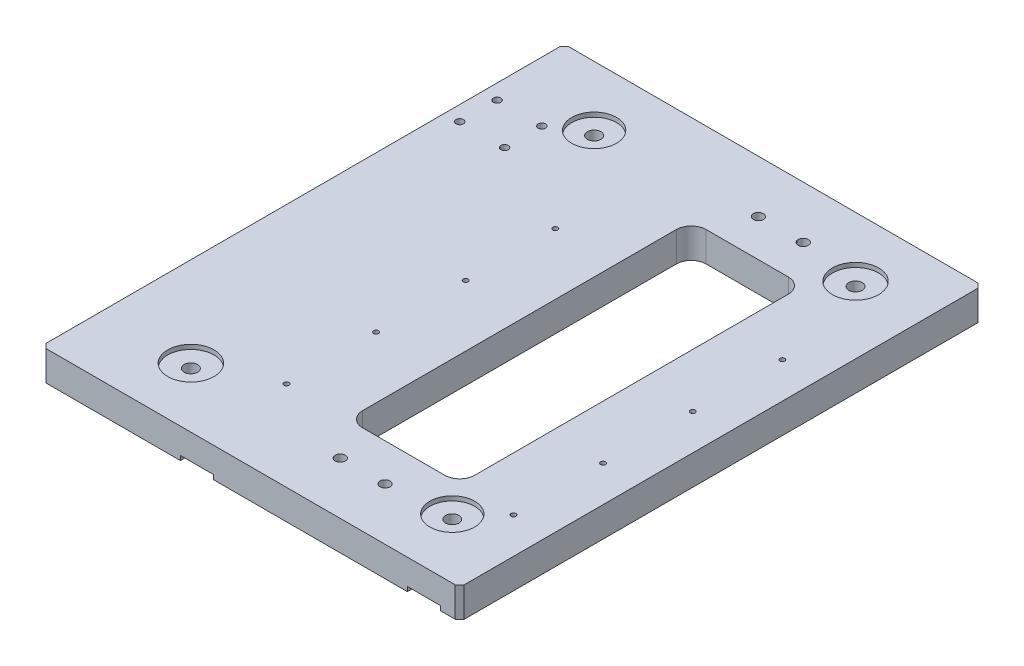
from build123d import *

# Parameters (mm, degrees)
BOSS_EXTRUDE1_DEPTH         = 350
CHAMFER1_SIZE               = 3
SKETCH2_W                   = 75
SKETCH2_H                   = 230
CUT_EXTRUDE1_DEPTH          = 395.884460879
FILLET1_R                   = 10
HOLE1_D                     = 9
HOLE1_DEPTH                 = 17
HOLE1_CBORE_D               = 15
HOLE1_CBORE_DEPTH           = 10.5
M4_TAPPED_HOLE1_D           = 3.3
M4_TAPPED_HOLE1_CSINK_D     = 4.05
M4_TAPPED_HOLE1_CSINK_ANGLE = 90
HOLE2_D                     = 31
HOLE2_DEPTH                 = 3
HOLE3_D                     = 30
HOLE3_DEPTH                 = 3
M8_TAPPED_HOLE1_D           = 6.8
M6_TAPPED_HOLE2_D           = 5


with BuildPart() as part:
    # Sketch1 → Boss-Extrude1 (new body)
    with BuildSketch(Plane.XY):
        Polygon((16.751856783, 37.381546135), (146.751856783, 37.381546135), (146.751856783, 40.381546135), (168.751856783, 40.381546135), (168.751856783, 37.381546135), (181.751856783, 37.381546135), (181.751856783, 57.381546135), (-98.248143217, 57.381546135), (-98.248143217, 37.381546135), (-5.248143217, 37.381546135), (-5.248143217, 40.381546135), (16.751856783, 40.381546135), align=None)
    extrude(amount=BOSS_EXTRUDE1_DEPTH)

    # Chamfer1
    chamfer1_edges = [part.edges().sort_by_distance(p)[0] for p in [
        (181.751856783, 47.381546135, 0),
        (-98.248143217, 47.381546135, 0),
        (181.751856783, 47.381546135, 350),
        (-98.248143217, 47.381546135, 350),
    ]]
    chamfer(chamfer1_edges, length=CHAMFER1_SIZE)

    # Sketch2 → Cut-Extrude1 (cut, through all)
    with BuildSketch(Plane.XZ.offset(-37.381546135)):
        with Locations((84.251856783, 175)):
            Rectangle(SKETCH2_W, SKETCH2_H)
    extrude(amount=-CUT_EXTRUDE1_DEPTH, mode=Mode.SUBTRACT)

    # Fillet1
    fillet1_edges = [part.edges().sort_by_distance(p)[0] for p in [
        (46.751856783, 47.381546135, 60),
        (46.751856783, 47.381546135, 290),
        (121.751856783, 47.381546135, 290),
        (121.751856783, 47.381546135, 60),
    ]]
    fillet(fillet1_edges, radius=FILLET1_R)

    # Hole1
    with Locations(Plane(origin=(0, 37.381546135, 0), x_dir=(-1, 0, 0), z_dir=(0, -1, 0))):
        with Locations((38.248143217, -310), (-136.751856783, -310), (-136.751856783, -40), (38.248143217, -40)):
            CounterBoreHole(HOLE1_D / 2, HOLE1_CBORE_D / 2, HOLE1_CBORE_DEPTH, depth=HOLE1_DEPTH)

    # M4 Tapped Hole1 (through all)
    with Locations(Plane(origin=(0, 40.381546135, 0), x_dir=(-1, 0, 0), z_dir=(0, -1, 0))):
        with Locations((-5.751856783, -290), (-5.751856783, -230), (-5.751856783, -170), (-157.751856783, -170), (-157.751856783, -230), (-157.751856783, -290), (-5.751856783, -110), (-157.751856783, -110)):
            CounterSinkHole(M4_TAPPED_HOLE1_D / 2, M4_TAPPED_HOLE1_CSINK_D / 2, counter_sink_angle=M4_TAPPED_HOLE1_CSINK_ANGLE)

    # Hole2
    with Locations(Plane(origin=(0, 57.381546135, 0), x_dir=(1, 0, 0), z_dir=(0, 1, 0))):
        with Locations((-38.248143217, -310), (136.751856783, -40)):
            Hole(HOLE2_D / 2, depth=HOLE2_DEPTH)

    # Hole3
    with Locations(Plane(origin=(0, 57.381546135, 0), x_dir=(1, 0, 0), z_dir=(0, 1, 0))):
        with Locations((-38.248143217, -40), (136.751856783, -310)):
            Hole(HOLE3_D / 2, depth=HOLE3_DEPTH)

    # M8 Tapped Hole1 (through all)
    with Locations(Plane(origin=(0, 57.381546135, 0), x_dir=(1, 0, 0), z_dir=(0, 1, 0))):
        with Locations((96.751856783, -315), (66.751856783, -315), (96.751856783, -35), (66.751856783, -35)):
            Hole(M8_TAPPED_HOLE1_D / 2)

    # M6 Tapped Hole2 (through all)
    with Locations(Plane(origin=(0, 57.381546135, 0), x_dir=(1, 0, 0), z_dir=(0, 1, 0))):
        with Locations((-58.248143217, -80), (-58.248143217, -55), (-88.248143217, -55), (-88.248143217, -80)):
            Hole(M6_TAPPED_HOLE2_D / 2)


solid = part.part
